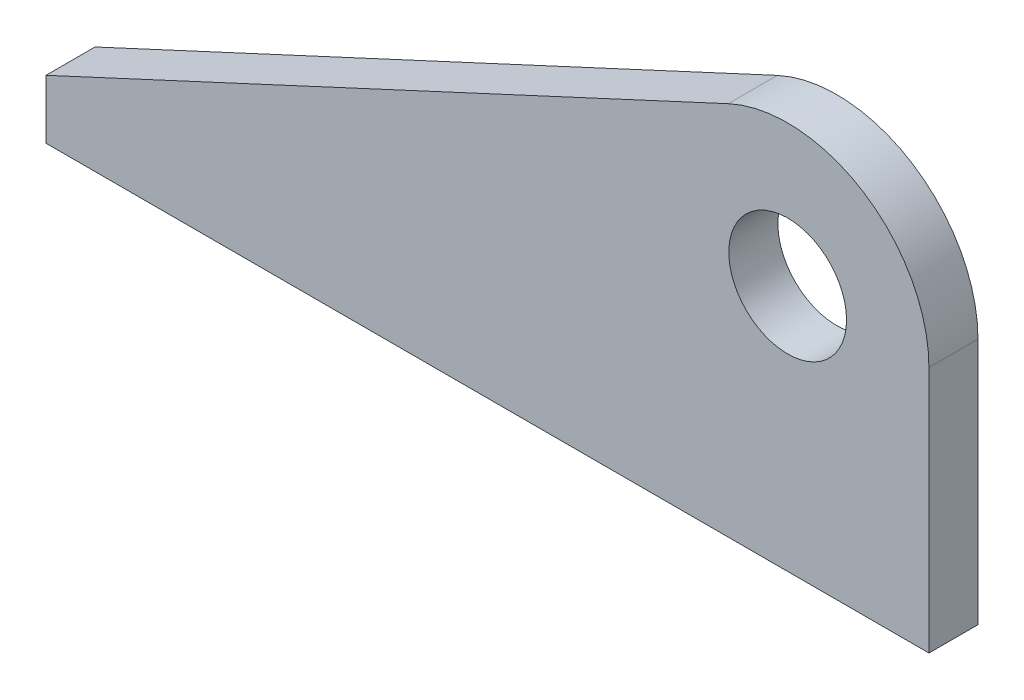
SolidWorks part; units mm, degrees
material "Q235"
ref_plane "Front Plane" through (0, 0, 0) normal (0, 0, 1) x (1, 0, 0)
ref_plane "Top Plane" through (0, 0, 0) normal (0, 1, 0) x (1, 0, 0)
ref_plane "Right Plane" through (0, 0, 0) normal (1, 0, 0) x (0, 0, -1)
sketch "Sketch1" plane through (0, 0, 0) normal (0, 0, 1) x (1, 0, 0)
  line L0 (0, 0) -> (0, 30)
  line L1 (0, 30) -> (347.6983, 191.3131)
  line L2 (450, 126) -> (450, 0)
  line L3 (450, 0) -> (0, 0)
  arc A0 (347.6983, 191.3131) -> (450, 126) centre (378, 126) cw
  circle A1 centre (378, 126) radius 30
  dimension "D2" = 72
  dimension "D6" = 60
  dimension "D1" = 378
  dimension "D3" = 126
  dimension "D4" = 30
  dimension "D5" = 126
extrude "Boss-Extrude1" add sketch "Sketch1" along normal blind 25
